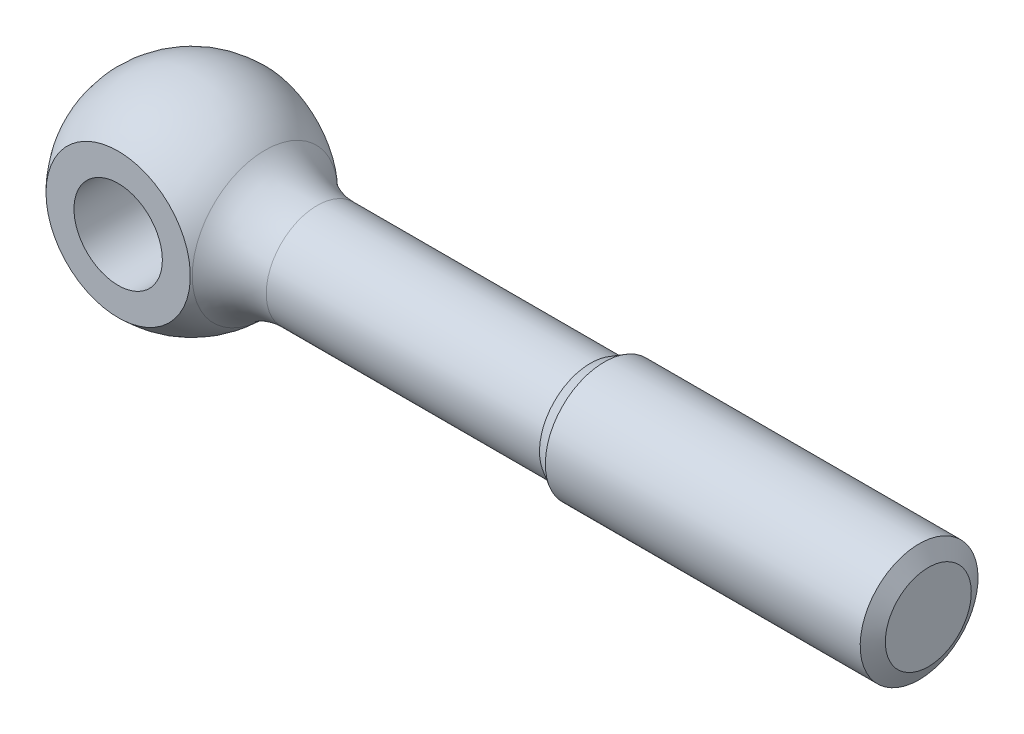
from build123d import *
from build123d.topology import SkipClean

# Parameters (mm, degrees)
CUT_EXTRUDE1_DEPTH      = 13.124356
CUT_EXTRUDE1_DEPTH_BACK = 13.124356
SKETCH4_R               = 3
CUT_EXTRUDE2_DEPTH      = 16.556349
CHAMFER1_SIZE           = 0.4
FILLET1_R               = 5


with BuildPart() as part:
    # Sketch1 → Boss-Revolve (revolve)
    with BuildSketch(Plane.XY):
        with BuildLine():
            Line((-7, 0), (7, 0))
            ThreePointArc((7, 0), (0, 7), (-7, 0))
        make_face()
    revolve(axis=Axis((-13.286843, 0, 0), (1, 0, 0)))

    # Sketch2 → Cut-Extrude1 (cut, two sides: drawn at the far end of the back side and taken through both)
    with SkipClean():  # the faces are left unmerged after this step: merging them gives an invalid solid
        with BuildSketch(Plane(origin=(0, 0, 0), x_dir=(0, 0, -1), z_dir=(1, 0, 0)).offset(-CUT_EXTRUDE1_DEPTH_BACK)):
            with BuildLine():
                Line((-5, 4.898979), (-5, -4.898979))
                ThreePointArc((-5, -4.898979), (-7, 0), (-5, 4.898979))
            make_face()
            with BuildLine():
                Line((5, 4.898979), (5, -4.898979))
                ThreePointArc((5, -4.898979), (7, 0), (5, 4.898979))
            make_face()
        extrude(amount=CUT_EXTRUDE1_DEPTH + CUT_EXTRUDE1_DEPTH_BACK, mode=Mode.SUBTRACT)

    # Sketch4 → Cut-Extrude2 (cut, through all)
    with SkipClean():  # the faces are left unmerged after this step: merging them gives an invalid solid
        with BuildSketch(Plane.XY.offset(5)):
            Circle(SKETCH4_R)
        extrude(amount=-CUT_EXTRUDE2_DEPTH, mode=Mode.SUBTRACT)

    # Sketch5 → Boss-Revolve1 (revolve)
    with SkipClean():  # the faces are left unmerged after this step: merging them gives an invalid solid
        with BuildSketch(Plane.XY, mode=Mode.PRIVATE) as boss_revolve1_sk:
            Polygon((3.469445, 3.45875), (3.469445, 0), (50, 0), (50, 4), (28, 4), (27.062528, 3.45875), align=None)
        revolve(boss_revolve1_sk.sketch.rotate(Axis((0, 0, 0), (1, 0, 0)), 180), axis=Axis((0, 0, 0), (1, 0, 0)))

    # Chamfer1
    chamfer1_edges = [part.edges().sort_by_distance(p)[0] for p in [
        (50, 4, 0),
    ]]
    chamfer(chamfer1_edges, length=CHAMFER1_SIZE)

    # Sketch6 → Cut-Revolve1 (revolve, cut)
    with SkipClean():  # the faces are left unmerged after this step: merging them gives an invalid solid
        with BuildSketch(Plane.XY, mode=Mode.PRIVATE) as cut_revolve1_sk:
            Polygon((49.375018, 4), (50.624982, 4), (50, 2.9175), align=None)
        revolve(cut_revolve1_sk.sketch.rotate(Axis((0, 0, 0), (1, 0, 0)), 180), axis=Axis((0, 0, 0), (1, 0, 0)), mode=Mode.SUBTRACT)

    # Fillet1
    fillet1_edges = [part.edges().sort_by_distance(p)[0] for p in [
        (6.085807, 0, -3.45875),
    ]]
    fillet(fillet1_edges, radius=FILLET1_R)


solid = part.part
